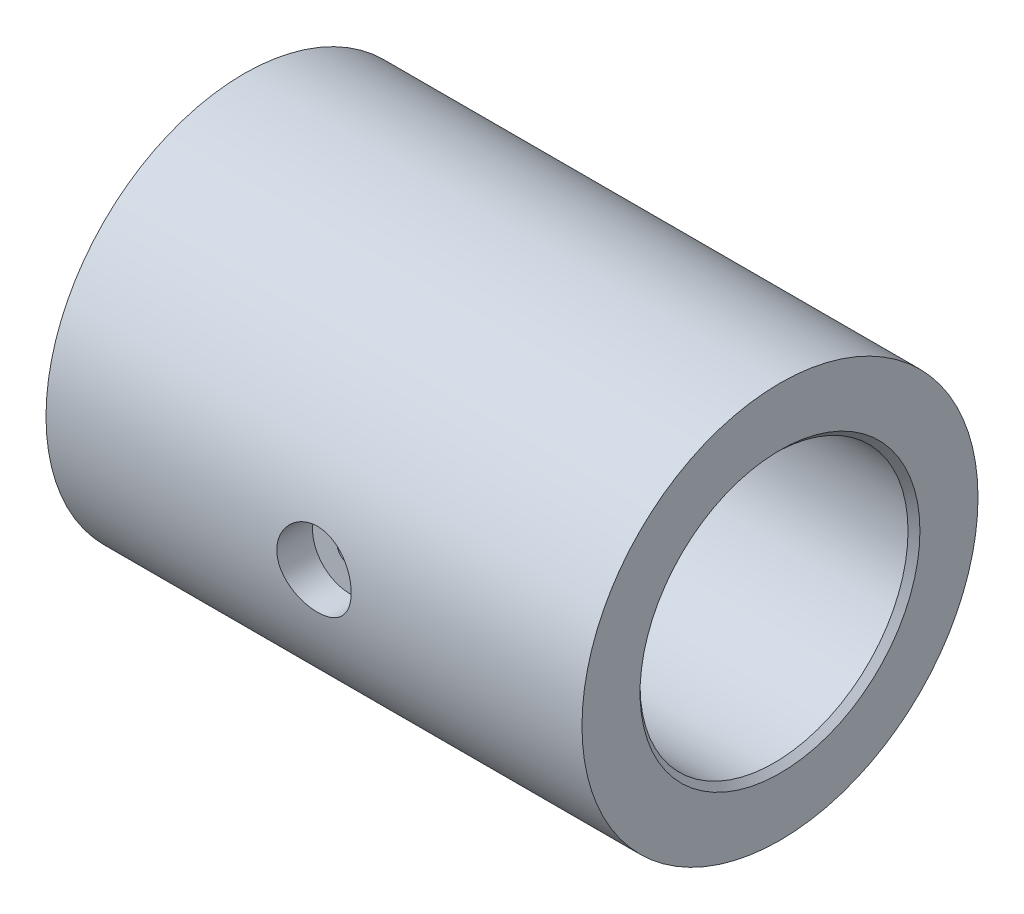
from build123d import *

# Parameters (mm, degrees)
SKETCH1_R              = 66.5
SKETCH1_R_2            = 45
BOSS_EXTRUDE1_DEPTH    = 90
M10_TAPPED_HOLE1_D     = 8.5
M10_TAPPED_HOLE1_DEPTH = 66.499
M10_TAPPED_HOLE1_TIP   = 2.553657631
SKETCH4_R              = 12.5
CUT_EXTRUDE1_DEPTH     = 12
CHAMFER1_SIZE          = 2


with BuildPart() as part:
    # Sketch1 → Boss-Extrude1 (new, symmetric)
    with BuildSketch(Plane(origin=(0, 0, 0), x_dir=(0, 0, -1), z_dir=(1, 0, 0))):
        with Locations(Location((0, 0, 0), (0, 0, 180))):
            Circle(SKETCH1_R)
        with Locations(Location((0, 0, 0), (0, 0, 180))):
            Circle(SKETCH1_R_2, mode=Mode.SUBTRACT)
    extrude(amount=BOSS_EXTRUDE1_DEPTH, both=True)

    # M10 Tapped Hole1
    with Locations(Plane.XY.offset(66.5)):
        with Locations((0, 0)):
            Hole(M10_TAPPED_HOLE1_D / 2, depth=M10_TAPPED_HOLE1_DEPTH)
            with Locations((0, 0, -(M10_TAPPED_HOLE1_DEPTH + M10_TAPPED_HOLE1_TIP / 2))):  # 118° drill point
                Cone(0, M10_TAPPED_HOLE1_D / 2, M10_TAPPED_HOLE1_TIP, mode=Mode.SUBTRACT)

    # Sketch4 → Cut-Extrude1 (cut)
    with BuildSketch(Plane.XY.offset(66.5)):
        Circle(SKETCH4_R)
    extrude(amount=-CUT_EXTRUDE1_DEPTH, mode=Mode.SUBTRACT)

    # Chamfer1
    chamfer1_edges = [part.edges().sort_by_distance(p)[0] for p in [
        (-90, 0, -45),
        (90, 0, -45),
    ]]
    chamfer(chamfer1_edges, length=CHAMFER1_SIZE)


solid = part.part
